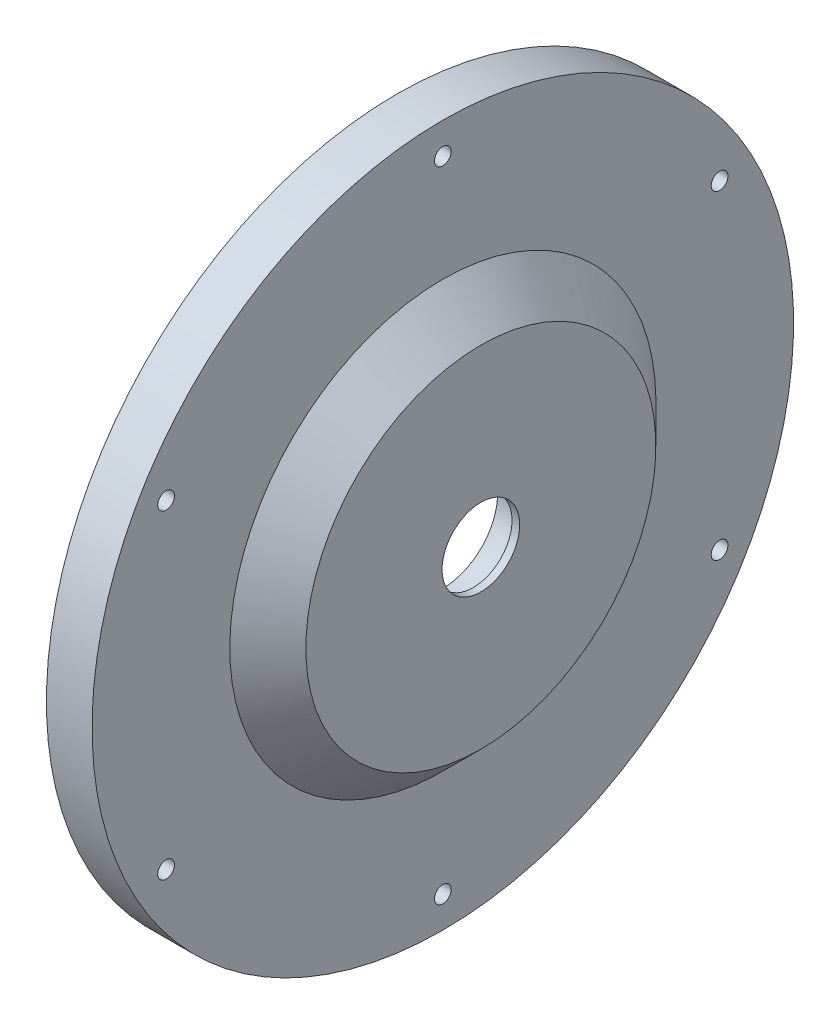
from build123d import *

# Parameters (mm, degrees)
SKETCH2_R          = 5.5
CUT_EXTRUDE1_DEPTH = 85


with BuildPart() as part:
    # Sketch1 → Revolve1 (revolve)
    with BuildSketch(Plane.XY):
        with BuildLine():
            Line((-25, 230.5), (-25, 140))
            Line((-25, 140), (0, 115))
            Line((0, 115), (0, 25.5))
            Line((0, 25.5), (-5, 25.5))
            Line((-5, 25.5), (-5, 35))
            ThreePointArc((-5, 35), (-5.292893219, 35.707106781), (-6, 36))
            Line((-6, 36), (-25, 36))
            Line((-25, 36), (-25, 52.5))
            Line((-25, 52.5), (-55, 82.5))
            Line((-55, 82.5), (-55, 205.5))
            Line((-55, 205.5), (-55, 215.5))
            Line((-55, 215.5), (-55, 230.5))
            Line((-55, 230.5), (-25, 230.5))
        make_face()
    revolve(axis=Axis((5, 0, 0), (-1, 0, 0)))

    # Sketch2 → Cut-Extrude1 (cut)
    with BuildSketch(Plane.ZY.offset(55)):
        with Locations(Location((0, 210, 0), (0, 0, 270))):
            Circle(SKETCH2_R)
        with Locations(Location((181.865334795, 105, 0), (0, 0, 270))):
            Circle(SKETCH2_R)
        with Locations(Location((181.865334795, -105, 0), (0, 0, 270))):
            Circle(SKETCH2_R)
        with Locations(Location((0, -210, 0), (0, 0, 270))):
            Circle(SKETCH2_R)
        with Locations(Location((-181.865334795, -105, 0), (0, 0, 270))):
            Circle(SKETCH2_R)
        with Locations(Location((-181.865334795, 105, 0), (0, 0, 270))):
            Circle(SKETCH2_R)
    extrude(amount=-CUT_EXTRUDE1_DEPTH, mode=Mode.SUBTRACT)


solid = part.part
